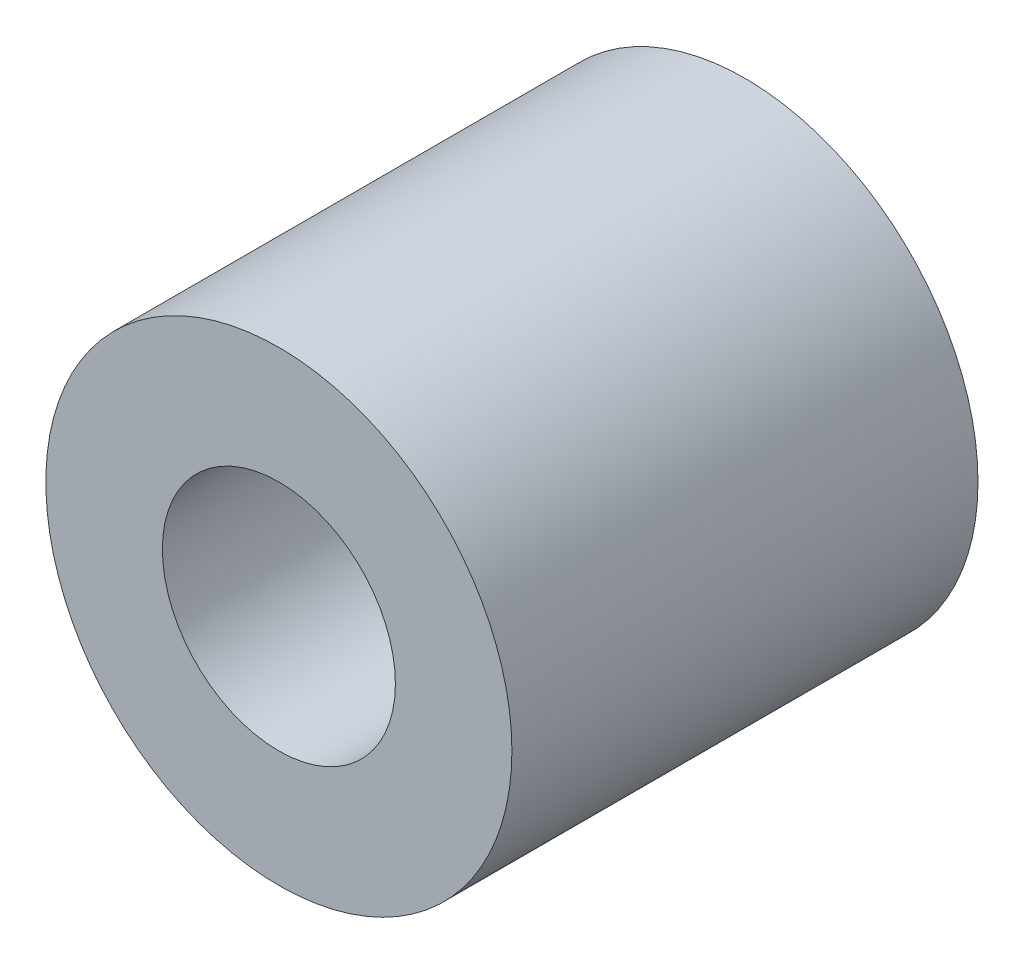
from build123d import *

# Parameters (mm, degrees)
SKETCH_1_R          = 30
EXTRUDE_1_DEPTH     = 60
SKETCH_2_R          = 7
CUT_EXTRUDE_1_DEPTH = 74.484692283
SKETCH_3_R          = 15
CUT_EXTRUDE_2_DEPTH = 30


with BuildPart() as part:
    # 草图1 → 凸台-拉伸1 (new body)
    with BuildSketch(Plane.XY):
        Circle(SKETCH_1_R)
    extrude(amount=EXTRUDE_1_DEPTH)

    # 草图2 → 切除-拉伸1 (cut, through all)
    with BuildSketch(Plane.XY.offset(60)):
        Circle(SKETCH_2_R)
    extrude(amount=-CUT_EXTRUDE_1_DEPTH, mode=Mode.SUBTRACT)

    # 草图3 → 切除-拉伸2 (cut)
    with BuildSketch(Plane.XY.offset(60)):
        Circle(SKETCH_3_R)
    extrude(amount=-CUT_EXTRUDE_2_DEPTH, mode=Mode.SUBTRACT)


solid = part.part
